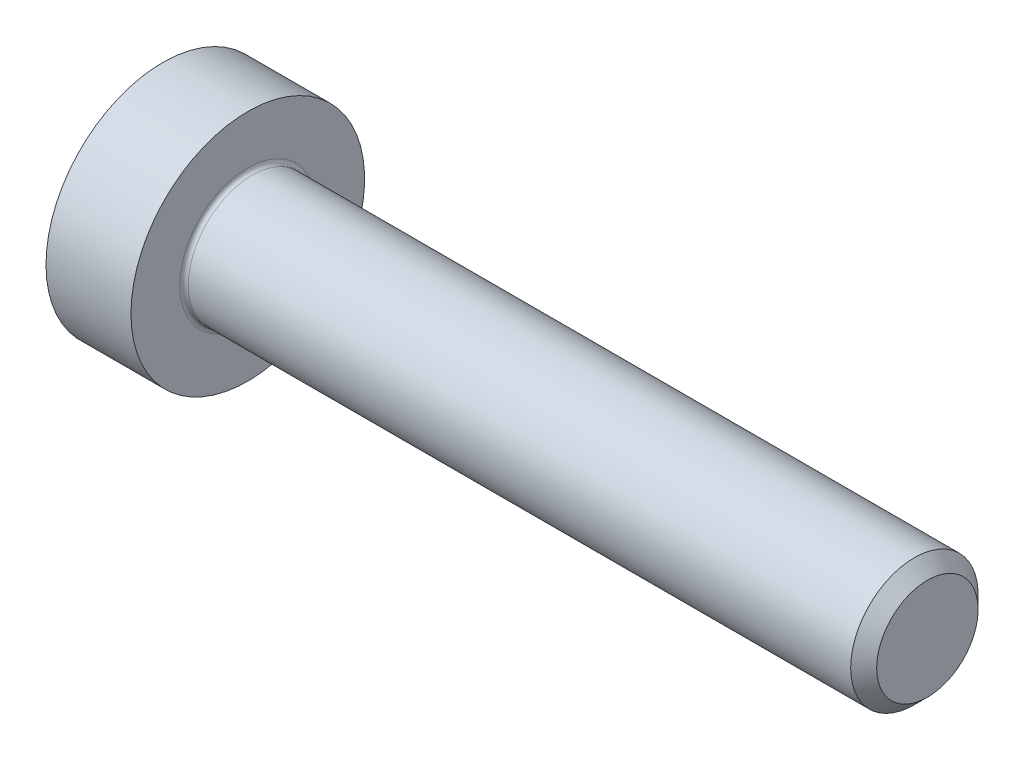
SolidWorks part; units mm, degrees
ref_plane "Front Plane" through (0, 0, 0) normal (0, 0, 1) x (1, 0, 0)
ref_plane "Top Plane" through (0, 0, 0) normal (0, 1, 0) x (1, 0, 0)
ref_plane "Right Plane" through (0, 0, 0) normal (1, 0, 0) x (0, 0, -1)
sketch "Sketch1" plane through (0, 0, 0) normal (0, 0, 1) x (1, 0, 0)
  line L0 (-2, 0) -> (-2, 2.75)
  line L1 (-2, 2.75) -> (0, 2.75)
  line L2 (0, 2.75) -> (0, 1.6)
  line L3 (0.1, 1.5) -> (15.6935, 1.5)
  line L4 (15.6935, 1.5) -> (16, 1.1935)
  line L5 (16, 1.1935) -> (16, 0)
  line L6 (16, 0) -> (-2, 0)
  line L7 (16, 0) -> (-2, 0) construction
  arc A0 (0, 1.6) -> (0.1, 1.5) centre (0.1, 1.6) ccw
revolve "Revolve1" add sketch "Sketch1" angle 360 about L7
cosmetic thread "Cosmetic Thread1" parameters "D1"=15.5, "D2"=2.387
sketch "Sketch2" plane through (0, 0, 0) normal (0, 0, 1) x (1, 0, 0)
  line L0 (-2, 0) -> (-2, 1)
  line L1 (-2, 1) -> (-0.5, 1)
  line L2 (-0.5, 1) -> (-0.136, 0)
  line L3 (-0.136, 0) -> (-2, 0)
  line L4 (0, 0) -> (-2, 0) construction
revolve "Cut-Revolve1" cut sketch "Sketch2" angle 360 about L4
ref_plane "Plane1" through (-2, 0, 0) normal (1, 0, 0) x (0, 0, -1)
sketch "Sketch3" plane through (-2, 0, 0) normal (1, 0, 0) x (0, 0, -1)
  line L0 (-1, 0.5774) -> (-1, -0.5774)
  line L1 (-1, -0.5774) -> (0, -1.1547)
  line L2 (0, -1.1547) -> (1, -0.5774)
  line L3 (1, -0.5774) -> (1, 0.5774)
  line L4 (1, 0.5774) -> (0, 1.1547)
  line L5 (0, 1.1547) -> (-1, 0.5774)
extrude "Cut-Extrude1" cut sketch "Sketch3" along normal blind 1.5
